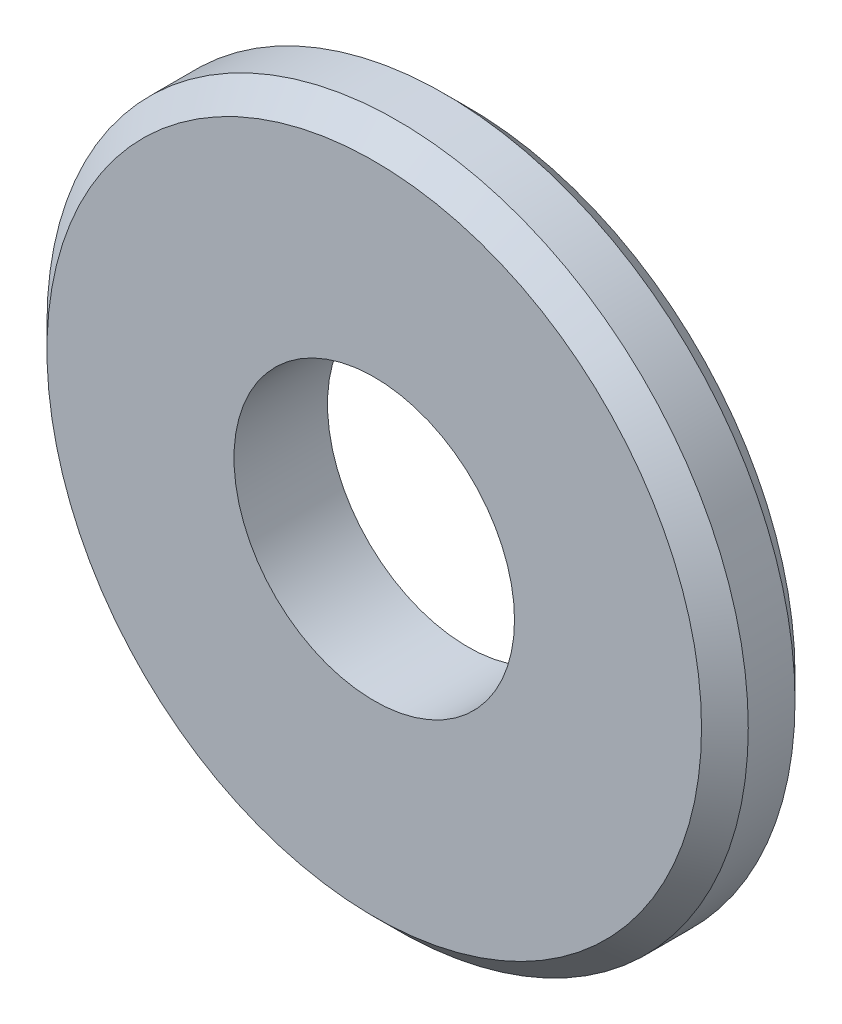
SolidWorks part; units mm, degrees
material "POM 白色"
ref_plane "Front Plane" through (0, 0, 0) normal (0, 0, 1) x (1, 0, 0)
ref_plane "Top Plane" through (0, 0, 0) normal (0, 1, 0) x (1, 0, 0)
ref_plane "Right Plane" through (0, 0, 0) normal (1, 0, 0) x (0, 0, -1)
sketch "Sketch1" plane through (0, 0, 0) normal (0, 0, 1) x (1, 0, 0)
  circle A0 centre (0, 0) radius 7.5
  circle A1 centre (0, 0) radius 3
  dimension "D1" = 6
  dimension "D2" = 15
extrude "Boss-Extrude1" add sketch "Sketch1" along normal blind 2
chamfer "Chamfer1" distance 0.5 angle 45 2 edges at (7.5, 0, 0) (7.5, 0, 2)
